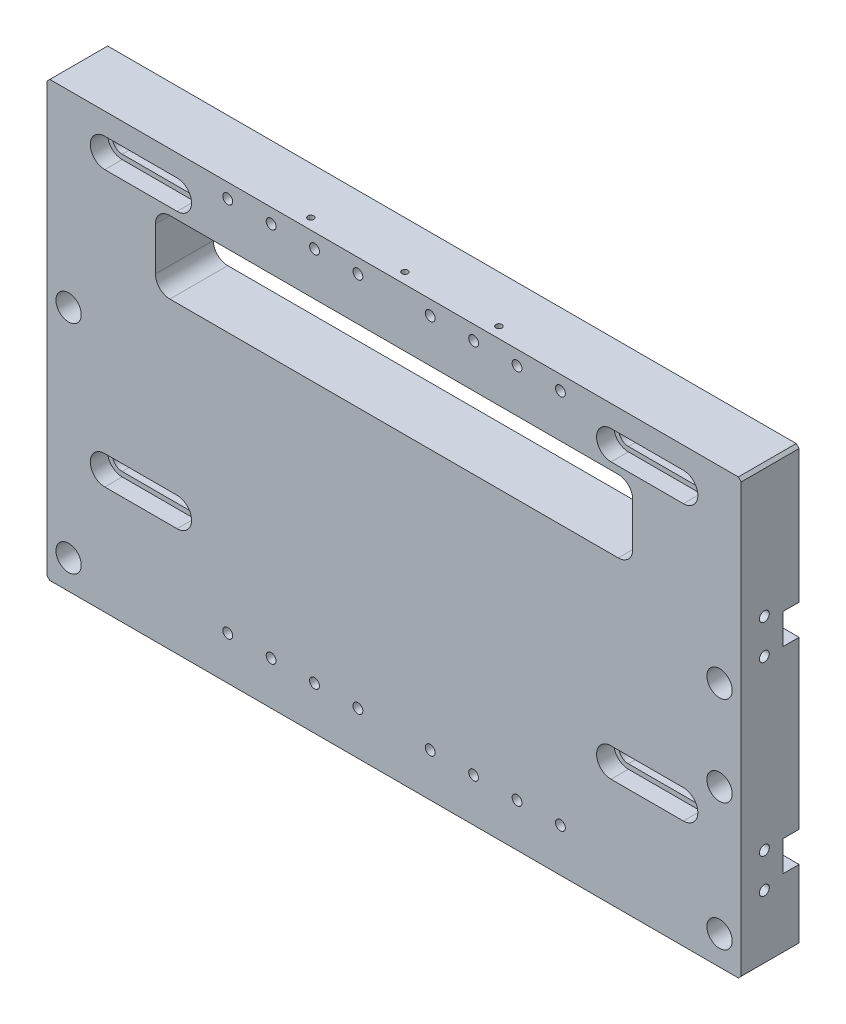
SolidWorks part; units mm, degrees
ref_plane "Front Plane" through (0, 0, 0) normal (0, 0, 1) x (1, 0, 0)
ref_plane "Top Plane" through (0, 0, 0) normal (0, 1, 0) x (1, 0, 0)
ref_plane "Right Plane" through (0, 0, 0) normal (1, 0, 0) x (0, 0, -1)
sketch "Sketch1" plane through (0, 0, 0) normal (0, 0, 1) x (1, 0, 0)
  line L1 (-240, 150) -> (240, 150)
  line L2 (-240, 150) -> (-240, -150)
  line L3 (-240, -150) -> (240, -150)
  line L4 (240, 150) -> (240, -150)
  line L5 (-240, 150) -> (240, -150) construction
  line L6 (-240, -150) -> (240, 150) construction
  point P0 (0, 0)
  dimension "D1" = 480
  dimension "D2" = 300
extrude "Boss-Extrude1" add sketch "Sketch1" along normal mid plane 40
sketch "Sketch2" plane through (0, 0, 20) normal (0, 0, 1) x (1, 0, 0)
  line L0 (0, 150) -> (0, -150) construction
  line L1 (240, 150) -> (-240, 150) construction
  line L2 (-240, -150) -> (240, -150) construction
  line L4 (-155, 110) -> (155, 110)
  line L5 (-165, 100) -> (-165, 70)
  line L6 (-155, 60) -> (155, 60)
  line L7 (165, 100) -> (165, 70)
  line L8 (-165, 110) -> (165, 60) construction
  line L9 (-165, 60) -> (165, 110) construction
  arc A0 (155, 60) -> (165, 70) centre (155, 70) ccw
  arc A1 (155, 110) -> (165, 100) centre (155, 100) cw
  arc A2 (-155, 110) -> (-165, 100) centre (-155, 100) ccw
  arc A3 (-165, 70) -> (-155, 60) centre (-155, 70) ccw
  point P6 (0, 85)
  dimension "D4" = 10
  dimension "D1" = 50
  dimension "D2" = 40
  dimension "D3" = 330
extrude "Cut-Extrude1" cut sketch "Sketch2" against normal through all
hole_wizard "Hole size per socket head cap screw type2" positions "Sketch4" profile "Sketch3" counterbore size "M16" standard "Gb" end condition through all
sketch "Sketch4" plane through (0, 0, -20) normal (0, 0, -1) x (-1, 0, 0)
  line L0 (0, 150) -> (0, -150) construction
  line L1 (-240, 150) -> (240, 150) construction
  line L2 (240, -150) -> (-240, -150) construction
  line L4 (-240, 0) -> (240, 0) construction
  line L5 (-240, -150) -> (-240, 150) construction
  line L6 (240, 150) -> (240, -150) construction
  point P0 (-225, 20)
  point P1 (225, 20)
  point P3 (225, -130)
  point P5 (-225, -130)
  point P22 (-225, -42)
  dimension "D1" = 450
  dimension "D2" = 150
  dimension "D3" = 20
  dimension "D4" = 88
sketch "Sketch3" plane through (225, 20, -20) normal (1, 0, 0) x (0, 1, 0)
  line L0 (0, 0) -> (0, 40)
  line L1 (0, 40) -> (8.75, 40)
  line L3 (8.75, 40) -> (8.75, 17.5)
  line L4 (8.75, 17.5) -> (13, 17.5)
  line L5 (13, 17.5) -> (13, 0)
  line L7 (13, 0) -> (0, 0)
  line L11 (0, -6.35) -> (0, 107.95) construction
  dimension "通孔孔直径" = 17.5
  dimension "通孔孔深度" = 40
  dimension "柱形沉头孔直径" = 26
  dimension "柱形沉头孔深度" = 17.5
hole_wizard "CBORE for M12 Hex Socket Head Cap Screw1" positions "Sketch6" profile "Sketch5" counterbore size "M12" standard "Iso" end condition through all
sketch "Sketch6" plane through (0, 0, 20) normal (0, 0, 1) x (1, 0, 0)
  line L0 (0, 150) -> (0, -150) construction
  line L1 (240, 150) -> (-240, 150) construction
  line L2 (-240, -150) -> (240, -150) construction
  point P1 (-200, 125)
  point P3 (200, 125)
  point P20 (-200, -65)
  point P22 (200, -65)
  dimension "D1" = 400
  dimension "D2" = 25
  dimension "D3" = 190
sketch "Sketch5" plane through (-200, 125, 20) normal (1, 0, 0) x (0, -1, 0)
  line L0 (0, 0) -> (0, 40)
  line L1 (0, 40) -> (6.75, 40)
  line L3 (6.75, 40) -> (6.75, 12)
  line L4 (6.75, 12) -> (10, 12)
  line L5 (10, 12) -> (10, 0)
  line L7 (10, 0) -> (0, 0)
  line L11 (0, -6.35) -> (0, 107.95) construction
  dimension "通孔孔直径" = 13.5
  dimension "通孔孔深度" = 40
  dimension "柱形沉头孔直径" = 20
  dimension "柱形沉头孔深度" = 12
sketch "Sketch7" plane through (-240, 0, 0) normal (-1, 0, 0) x (0, 0, 1)
  line L0 (-20, 150) -> (-20, -150) construction
  line L1 (-20, -101) -> (-9, -101)
  line L2 (-20, -101) -> (-20, -80)
  line L3 (-20, -80) -> (-9, -80)
  line L4 (-9, -101) -> (-9, -80)
  line L5 (20, -150) -> (-20, -150) construction
  line L6 (-20, 35) -> (-9, 35)
  line L7 (-20, 35) -> (-20, 56)
  line L8 (-20, 56) -> (-9, 56)
  line L9 (-9, 35) -> (-9, 56)
  dimension "D1" = 21
  dimension "D2" = 11
  dimension "D3" = 49
  dimension "D4" = 115
extrude "Cut-Extrude2" cut sketch "Sketch7" against normal through all
hole_wizard "M5 Tapped Hole1" positions "Sketch9" profile "Sketch8" tap size "M5" standard "GB"
sketch "Sketch9" plane through (0, 150, 0) normal (0, 1, 0) x (-1, 0, 0)
  line L0 (0, -20) -> (0, 20) construction
  line L1 (-240, -20) -> (240, -20) construction
  line L2 (-240, 20) -> (240, 20) construction
  point P1 (0, 12.5)
  point P3 (-65, 12.5)
  point P5 (65, 12.5)
  dimension "D1" = 130
  dimension "D2" = 7.5
sketch "Sketch8" plane through (0, 150, 12.5) normal (1, 0, 0) x (0, 0, 1)
  line L0 (0, 0) -> (0, 13.6618)
  line L1 (0, 13.6618) -> (2.1, 12.4)
  line L2 (2.1, 12.4) -> (2.1, 0)
  line L5 (2.1, 0) -> (0, 0)
  line L10 (0, 13.6618) -> (-2.1, 12.4) construction
  line L11 (0, -6.35) -> (0, 107.95) construction
  dimension "螺纹孔钻头直径" = 4.2
  dimension "螺纹孔钻头深度" = 12.4
  dimension "导头角度" = 118
cosmetic thread "Cosmetic Thread1" parameters "D1"=10, "D2"=5
cosmetic thread "Cosmetic Thread2" parameters "D1"=10, "D2"=5
cosmetic thread "Cosmetic Thread3" parameters "D1"=10, "D2"=5
sketch "Sketch14" plane through (0, 0, 8) normal (0, 0, 1) x (1, 0, 0)
  line L0 (-200, 125) -> (-150, 125) construction
  line L1 (-200, 131.75) -> (-150, 131.75)
  line L2 (-200, 118.25) -> (-150, 118.25)
  line L3 (-200, -65) -> (-150, -65) construction
  line L4 (-200, -58.25) -> (-150, -58.25)
  line L5 (-200, -71.75) -> (-150, -71.75)
  line L6 (200, -65) -> (150, -65) construction
  line L7 (200, -71.75) -> (150, -71.75)
  line L8 (200, -58.25) -> (150, -58.25)
  line L9 (200, 125) -> (150, 125) construction
  line L10 (200, 118.25) -> (150, 118.25)
  line L11 (200, 131.75) -> (150, 131.75)
  arc A0 (-200, 131.75) -> (-200, 118.25) centre (-200, 125) ccw
  arc A1 (-150, 118.25) -> (-150, 131.75) centre (-150, 125) ccw
  circle A2 centre (-200, 125) radius 6.75 construction
  arc A3 (-200, -58.25) -> (-200, -71.75) centre (-200, -65) ccw
  arc A4 (-150, -71.75) -> (-150, -58.25) centre (-150, -65) ccw
  arc A5 (200, -71.75) -> (200, -58.25) centre (200, -65) ccw
  arc A6 (150, -58.25) -> (150, -71.75) centre (150, -65) ccw
  arc A7 (200, 118.25) -> (200, 131.75) centre (200, 125) ccw
  arc A8 (150, 131.75) -> (150, 118.25) centre (150, 125) ccw
  point P2 (-175, 125)
  point P13 (-175, -65)
  point P18 (175, -65)
  point P26 (175, 125)
  dimension "D1" = 50
extrude "Cut-Extrude5" cut sketch "Sketch14" against normal blind 100
sketch "Sketch15" plane through (0, 0, 20) normal (0, 0, 1) x (1, 0, 0)
  line L0 (-200, 125) -> (-150, 125) construction
  line L1 (-200, 135) -> (-150, 135)
  line L2 (-200, 115) -> (-150, 115)
  line L3 (-200, -65) -> (-150, -65) construction
  line L4 (-200, -55) -> (-150, -55)
  line L5 (-200, -75) -> (-150, -75)
  line L6 (200, -65) -> (150, -65) construction
  line L7 (200, -75) -> (150, -75)
  line L8 (200, -55) -> (150, -55)
  line L9 (200, 125) -> (150, 125) construction
  line L10 (200, 115) -> (150, 115)
  line L11 (200, 135) -> (150, 135)
  arc A0 (-200, 135) -> (-200, 115) centre (-200, 125) ccw
  arc A1 (-150, 115) -> (-150, 135) centre (-150, 125) ccw
  circle A2 centre (-200, 125) radius 10 construction
  arc A3 (-200, -55) -> (-200, -75) centre (-200, -65) ccw
  arc A4 (-150, -75) -> (-150, -55) centre (-150, -65) ccw
  arc A5 (200, -75) -> (200, -55) centre (200, -65) ccw
  arc A6 (150, -55) -> (150, -75) centre (150, -65) ccw
  arc A7 (200, 115) -> (200, 135) centre (200, 125) ccw
  arc A8 (150, 135) -> (150, 115) centre (150, 125) ccw
  point P3 (-175, 125)
  point P13 (-175, -65)
  point P18 (175, -65)
  point P26 (175, 125)
  dimension "D1" = 50
extrude "Cut-Extrude6" cut sketch "Sketch15" against normal blind 12
chamfer "Chamfer1" distance 2 angle 45 4 edges at (-240, 150, 0) (240, 150, 0) (240, -150, 0) (-240, -150, 0)
hole_wizard "M8 Tapped Hole1" positions "Sketch19" profile "Sketch18" tap size "M8" standard "Gb"
sketch "Sketch19" plane through (0, 0, 20) normal (0, 0, 1) x (1, 0, 0)
  line L0 (-238, -150) -> (238, -150) construction
  line L1 (238, 150) -> (-238, 150) construction
  line L3 (0, -150) -> (0, 155.01) construction
  point P8 (55, 140)
  point P11 (-55, -120)
  point P20 (55, -120)
  point P23 (-55, 140)
  point P72 (-25, 140)
  point P74 (25, 140)
  point P76 (-85, 140)
  point P78 (85, 140)
  point P80 (-25, -120)
  point P82 (-85, -120)
  point P84 (85, -120)
  point P86 (25, -120)
  point P87 (-115, -120)
  point P91 (115, -120)
  point P99 (-115, 140)
  point P103 (115, 140)
  dimension "D1" = 30
  dimension "D2" = 10
  dimension "D3" = 30
  dimension "D4" = 50
  dimension "D5" = 30
  dimension "D6" = 30
  dimension "D7" = 30
  dimension "D9" = 30
sketch "Sketch18" plane through (55, 140, 20) normal (1, 0, 0) x (0, -1, 0)
  line L0 (0, 0) -> (0, 21.7929)
  line L1 (0, 21.7929) -> (3.4, 19.75)
  line L2 (3.4, 19.75) -> (3.4, 0)
  line L5 (3.4, 0) -> (0, 0)
  line L10 (0, 21.7929) -> (-3.4, 19.75) construction
  line L11 (0, -6.35) -> (0, 107.95) construction
  dimension "螺纹孔钻头直径" = 6.8
  dimension "螺纹孔钻头深度" = 19.75
  dimension "导头角度" = 118
cosmetic thread "Cosmetic Thread13" parameters "D1"=16, "D2"=8
cosmetic thread "Cosmetic Thread14" parameters "D1"=16, "D2"=8
cosmetic thread "Cosmetic Thread15" parameters "D1"=16, "D2"=8
cosmetic thread "Cosmetic Thread18" parameters "D1"=16, "D2"=8
cosmetic thread "Cosmetic Thread19" parameters "D1"=16, "D2"=8
cosmetic thread "Cosmetic Thread20" parameters "D1"=16, "D2"=8
cosmetic thread "Cosmetic Thread21" parameters "D1"=16, "D2"=8
cosmetic thread "Cosmetic Thread22" parameters "D1"=16, "D2"=8
cosmetic thread "Cosmetic Thread23" parameters "D1"=16, "D2"=8
cosmetic thread "Cosmetic Thread24" parameters "D1"=16, "D2"=8
cosmetic thread "Cosmetic Thread25" parameters "D1"=16, "D2"=8
cosmetic thread "Cosmetic Thread26" parameters "D1"=16, "D2"=8
cosmetic thread "Cosmetic Thread44" parameters "D1"=16, "D2"=8
cosmetic thread "Cosmetic Thread46" parameters "D1"=16, "D2"=8
cosmetic thread "Cosmetic Thread55" parameters "D1"=16, "D2"=8
cosmetic thread "Cosmetic Thread56" parameters "D1"=16, "D2"=8
sketch "Sketch29" plane through (-240, 0, 0) normal (-1, 0, 0) x (0, 0, 1)
  line L0 (0, -148) -> (0, 51.8163) construction
  line L1 (-20, -148) -> (20, -148) construction
  circle A0 centre (0, -20) radius 11
  dimension "D1" = 22
  dimension "D2" = 20
extrude "Cut-Extrude7" cut sketch "Sketch29" against normal blind 130
sketch "Sketch30" plane through (-240, 0, 0) normal (-1, 0, 0) x (0, 0, 1)
  circle A0 centre (0, -20) radius 14.25
  dimension "D1" = 28.5
extrude "Cut-Extrude8" cut sketch "Sketch30" against normal blind 30
hole_wizard "M6 Tapped Hole2" positions "Sketch33" profile "Sketch31" tap size "M6" standard "Gb"
sketch "Sketch33" plane through (-240, 0, 0) normal (-1, 0, 0) x (0, 0, 1)
  line L0 (0, -20) -> (0, 12.5751) construction
  line L2 (0, -20) -> (25.0295, -20) construction
  circle A0 centre (0, -20) radius 21 construction
  point P27 (-10.5, -1.8135)
  point P29 (10.5, -1.8135)
  point P31 (10.5, -38.1865)
  point P33 (-10.5, -38.1865)
  dimension "D1" = 42
  dimension "D2" = 21
sketch "Sketch31" plane through (-240, -1.8135, -10.5) normal (0, 1, 0) x (0, 0, 1)
  line L0 (0, 0) -> (0, 16.5022)
  line L1 (0, 16.5022) -> (2.5, 15)
  line L2 (2.5, 15) -> (2.5, 0)
  line L5 (2.5, 0) -> (0, 0)
  line L10 (0, 16.5022) -> (-2.5, 15) construction
  line L11 (0, -6.35) -> (0, 107.95) construction
  dimension "螺纹孔钻头直径" = 5
  dimension "螺纹孔钻头深度" = 15
  dimension "导头角度" = 118
cosmetic thread "Cosmetic Thread47" parameters "D1"=12, "D2"=6
cosmetic thread "Cosmetic Thread48" parameters "D1"=12, "D2"=6
cosmetic thread "Cosmetic Thread49" parameters "D1"=12, "D2"=6
cosmetic thread "Cosmetic Thread50" parameters "D1"=12, "D2"=6
hole_wizard "M8 Tapped Hole2" positions "Sketch35" profile "Sketch34" tap size "M8" standard "Iso"
sketch "Sketch35" plane through (240, 0, 0) normal (1, 0, 0) x (0, 0, -1)
  point P0 (-4, -80.5)
  point P3 (-4, -104.5)
  point P6 (-4, 35.5)
  point P9 (-4, 59.5)
sketch "Sketch34" plane through (240, -80.5, 4) normal (0, 1, 0) x (0, 0, -1)
  line L0 (0, 0) -> (0, 24.2929)
  line L1 (0, 24.2929) -> (3.4, 22.25)
  line L2 (3.4, 22.25) -> (3.4, 0)
  line L5 (3.4, 0) -> (0, 0)
  line L10 (0, 24.2929) -> (-3.4, 22.25) construction
  line L11 (0, -6.35) -> (0, 107.95) construction
  dimension "螺纹孔钻头直径" = 6.8
  dimension "螺纹孔钻头深度" = 22.25
  dimension "导头角度" = 118
cosmetic thread "Cosmetic Thread51" parameters "D1"=16, "D2"=8
cosmetic thread "Cosmetic Thread52" parameters "D1"=16, "D2"=8
cosmetic thread "Cosmetic Thread53" parameters "D1"=16, "D2"=8
cosmetic thread "Cosmetic Thread54" parameters "D1"=16, "D2"=8
mirror "Mirror1" about plane through (0, 0, 0) normal (1, 0, 0) of "M8 Tapped Hole2"
